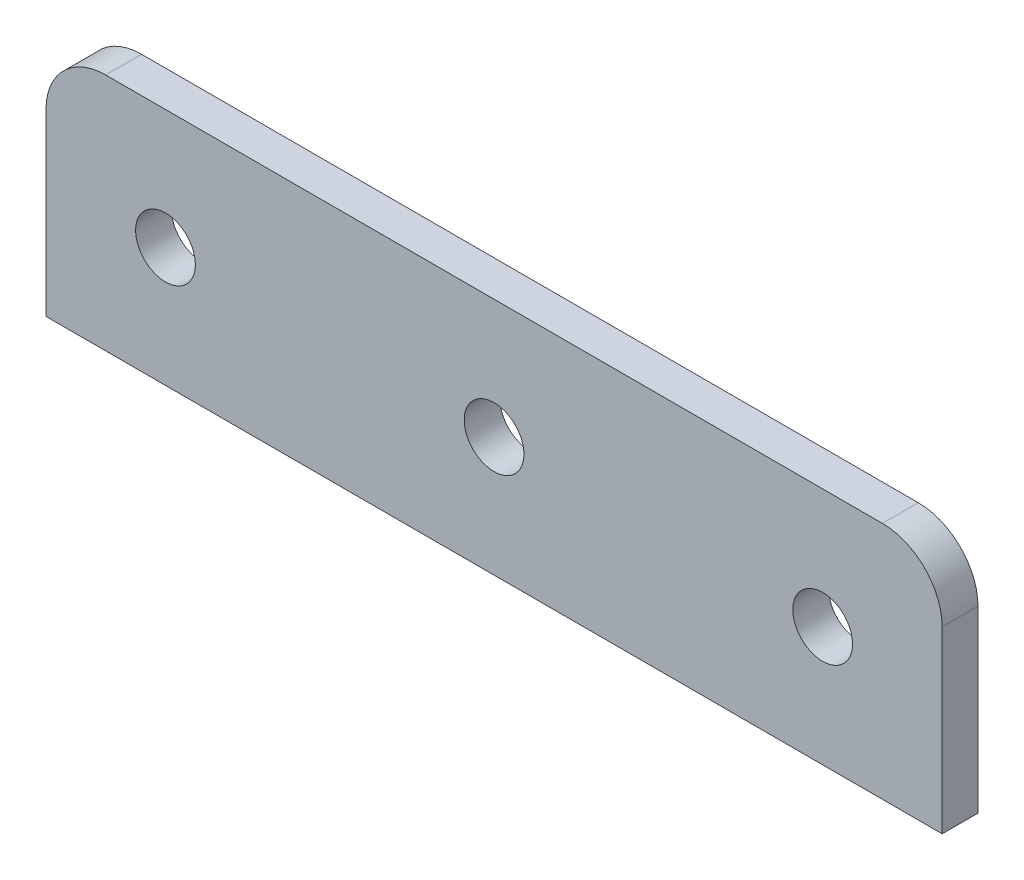
SolidWorks part; units mm, degrees
material "普通碳钢"
ref_plane "Front Plane" through (0, 0, 0) normal (0, 0, 1) x (1, 0, 0)
ref_plane "Top Plane" through (0, 0, 0) normal (0, 1, 0) x (1, 0, 0)
ref_plane "Right Plane" through (0, 0, 0) normal (1, 0, 0) x (0, 0, -1)
sketch "Sketch1" plane through (0, 0, 0) normal (0, 0, 1) x (1, 0, 0)
  line L1 (0, 0) -> (75, 0)
  line L2 (0, 0) -> (0, -20)
  line L3 (0, -20) -> (75, -20)
  line L4 (75, 0) -> (75, -20)
  line L5 (0, 0) -> (75, -20) construction
  line L6 (0, -20) -> (75, 0) construction
  circle A0 centre (10, -10) radius 2.5
  circle A2 centre (65, -10) radius 2.5
  circle A3 centre (37.5, -10) radius 2.5
  point P4 (37.5, -10)
  point P12 (37.5, -10)
  dimension "D3" = 5
  dimension "D1" = 20
  dimension "D2" = 75
  dimension "D4" = 27.5
  dimension "D5" = 27.5
  dimension "D6" = 10
extrude "Boss-Extrude1" add sketch "Sketch1" along normal blind 3
fillet "Fillet1" radius 5 2 edges at (75, 0, 1.5) (0, 0, 1.5)
